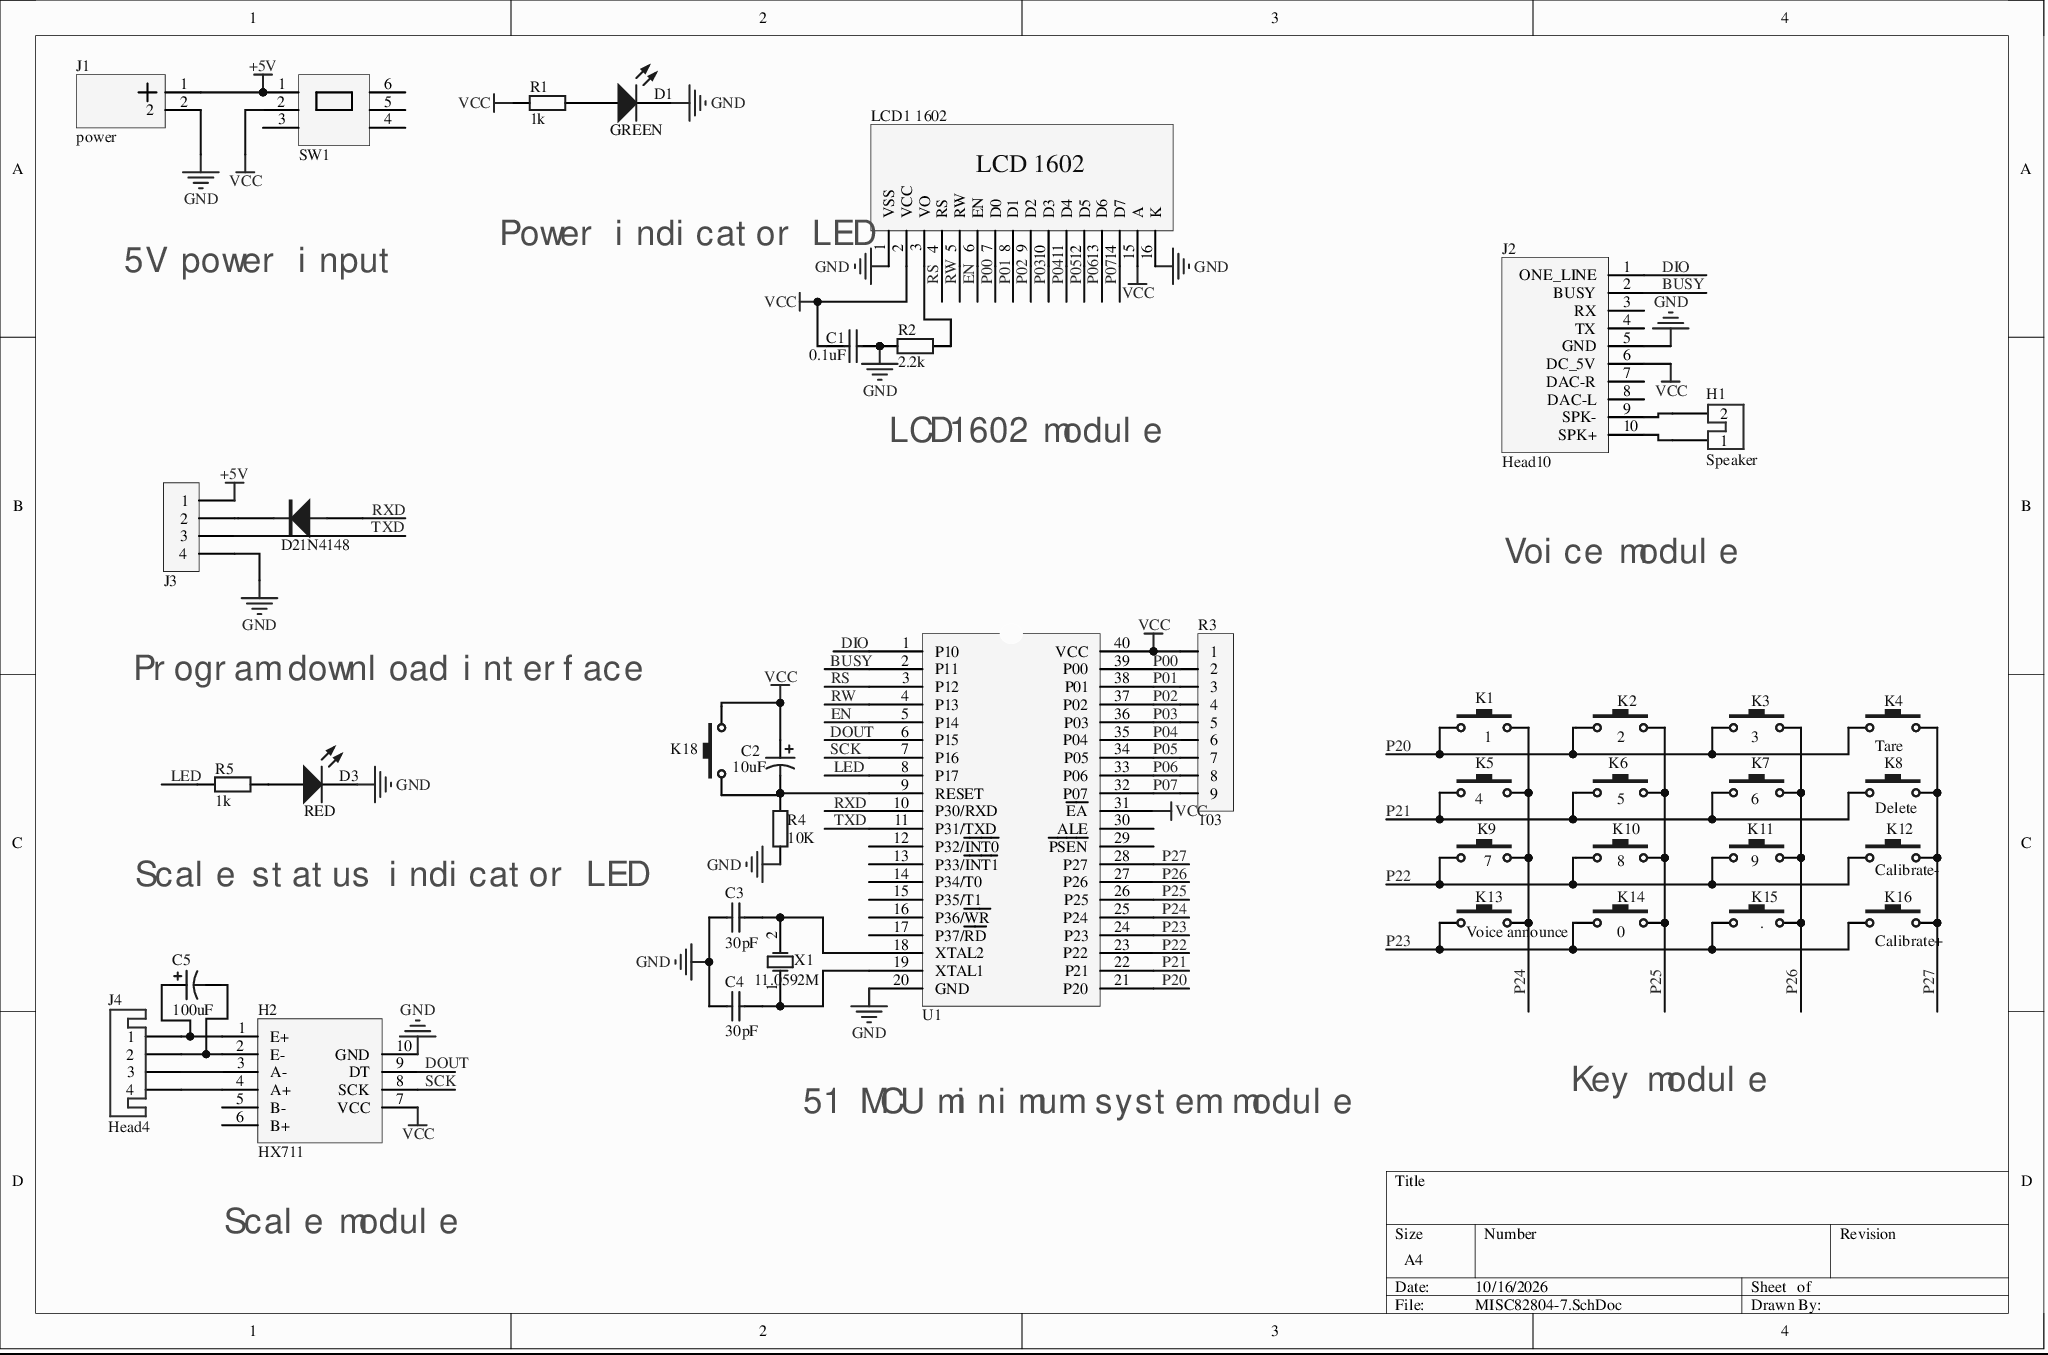
[diagram p0: MISC82804-7.SchDoc]
# Altium project MISC82804-4.PrjPcb
1 sheet, 40 parts. Net scope: global (net labels, ports and power ports of the same name join across sheets).
Board file: MISC82804.PcbDoc

## Sheet MISC82804-7.SchDoc
size A4; SheetNumber: 1; SheetTotal: 1

### Parts
C1  0.1uF  [CAP]
C2  10uF  [CAP_1]
C3  30pF  [CAP]
C4  30pF  [CAP]
C5  100uF  [CAP_2]
D1  GREEN  [LED_3MM_GREEN_1C-2A - duplicate]
D2  1N4148  [1N4148]
D3  RED  [LED_3MM_RED_1C-2A]
H1  Speaker  [609-2p-vr130]
H2  HX711  [hx711]
J1  power  [DC3.5 - me]
J2  Head10  [10PIN语音模块]
J3  SENSOR  [4PIN]  (value not drawn)
J4  Head4  [609-4p-vr130]
K1  1  [SW2]
K2  2  [SW2]
K3  3  [SW2]
K4  Tare  [SW2]
K5  4  [SW2]
K6  5  [SW2]
K7  6  [SW2]
K8  Delete  [SW2]
K9  7  [SW2]
K10  8  [SW2]
K11  9  [SW2]
K12  Calibrate-  [SW2]
K13  Voice announce  [SW2]
K14  0  [SW2]
K15  .  [SW2]
K16  Calibrate+  [SW2]
K18  KEY  [SW2]  (value not drawn)
LCD1  1602  [1602]
R1  1k  [电阻-RM7.5-C]
R2  2.2k  [电阻-RM7.5-C]
R3  103  [PAIRES]
R4  10K  [电阻-RM7.5-C]
R5  1k  [电阻-RM7.5-C]
SW1  SWT  [KEY-6]  (value not drawn)
U1  STC89C52  [C51]  (value not drawn)
X1  11.0592M  [12M]

### Nets
+5V: J1.1 J3.1 SW1.1
GND: C1.1 C3.1 C4.1 D1.2 D3.2 H2.10(GND) J1.2 J2.5(GND) J3.4 LCD1.1(VSS) LCD1.16(K) R2.2 R4.1 U1.20(GND)
VCC: C1.2 C2.1 H2.7(VCC) J2.6(DC_5V) K18.2 LCD1.2(VCC) LCD1.15(A) R1.1 R3.1 SW1.2 U1.31(~{EA}) U1.40(VCC)
BUSY: J2.2(BUSY) U1.2(P11)
DIO: J2.1(ONE_LINE) U1.1(P10)
DOUT: H2.9(DT) U1.6(P15)
EN: LCD1.6(EN) U1.5(P14)
LED: R5.1 U1.8(P17)
P00: LCD1.7(D0) R3.2 U1.39(P00)
P01: LCD1.8(D1) R3.3 U1.38(P01)
P02: LCD1.9(D2) R3.4 U1.37(P02)
P03: LCD1.10(D3) R3.5 U1.36(P03)
P04: LCD1.11(D4) R3.6 U1.35(P04)
P05: LCD1.12(D5) R3.7 U1.34(P05)
P06: LCD1.13(D6) R3.8 U1.33(P06)
P07: LCD1.14(D7) R3.9 U1.32(P07)
P20: K1.1 K2.1 K3.1 K4.1 U1.21(P20)
P21: K5.1 K6.1 K7.1 K8.1 U1.22(P21)
P22: K9.1 K10.1 K11.1 K12.1 U1.23(P22)
P23: K13.1 K14.1 K15.1 K16.1 U1.24(P23)
P24: K1.2 K5.2 K9.2 K13.2 U1.25(P24)
P25: K2.2 K6.2 K10.2 K14.2 U1.26(P25)
P26: K3.2 K7.2 K11.2 K15.2 U1.27(P26)
P27: K4.2 K8.2 K12.2 K16.2 U1.28(P27)
RS: LCD1.4(RS) U1.3(P12)
RW: LCD1.5(RW) U1.4(P13)
RXD: D2.1(A) U1.10(P30/RXD)
SCK: H2.8(SCK) U1.7(P16)
TXD: J3.3 U1.11(P31/TXD)
NetC2_2: C2.2 K18.1 R4.2 U1.9(RESET)
NetC3_2: C3.2 U1.18(XTAL2) X1.2(OSC2)
NetC4_2: C4.2 U1.19(XTAL1) X1.1(OSC1)
NetC5_1: C5.1 H2.1(E+) J4.1
NetC5_2: C5.2 H2.2(E-) J4.2
NetD1_1: D1.1 R1.2
NetD2_2: D2.2(K) J3.2
NetD3_1: D3.1 R5.2
NetH1_1: H1.1 J2.10(SPK+)
NetH1_2: H1.2 J2.9(SPK-)
NetH2_3: H2.3(A-) J4.3
NetH2_4: H2.4(A+) J4.4
NetLCD1_3: LCD1.3(VO) R2.1

Not connected (* = marked no-connect by the designer): H2 5(B-) 6(B+); J2 3(RX) 4(TX) 7(DAC-R) 8(DAC-L); SW1 3(2) 4(3) 5(4) 6(5); U1 12(P32/~{INT0}) 13(P33/~{INT1}) 14(P34/T0) 15(P35/T1) 16(P36/~{WR}) 17(P37/~{RD}) 29(~{PSEN}) 30(ALE)

### Notes on the sheet
- 5V power input
- (near LCD1) Power indicator LED
- LCD1602 module
- Voice module
- Program download interface
- Scale status indicator LED
- 51 MCU minimum system module
- Key module
- Scale module

### Library data of the parts
C1 = CAP: Capacitor
C2 C5 = CAP_2
C3 C4 = CAP
D1 D3 = LED
H1 = Head2
H2 = HX7111
J1 = DC5.5
J3 = CON4
K1-K16 = KEY
R1 R2 R4 R5 = Res
R3 = Header9
X1 = XTAL